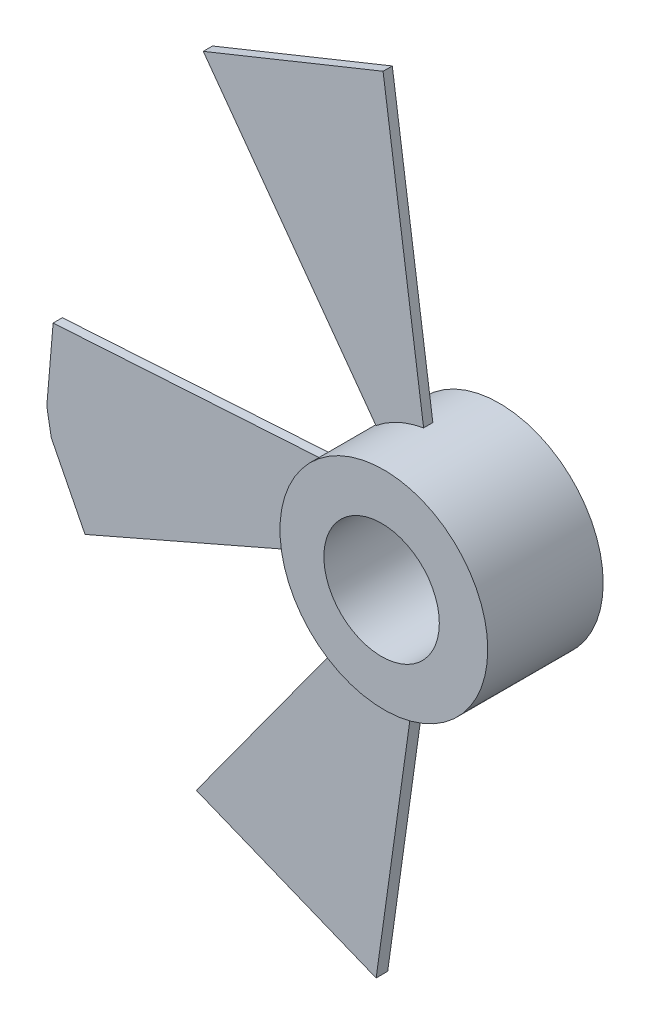
SolidWorks part; units mm, degrees
ref_plane "前视基准面" through (0, 0, 0) normal (0, 0, 1) x (1, 0, 0)
ref_plane "上视基准面" through (0, 0, 0) normal (0, 1, 0) x (1, 0, 0)
ref_plane "右视基准面" through (0, 0, 0) normal (1, 0, 0) x (0, 0, -1)
other "Configuration Table"
sketch "草图1" plane through (0, 0, 0) normal (0, 0, 1) x (1, 0, 0)
  line L0 (-10.9248, 55.6689) -> (-50.6906, 338.617)
  line L1 (-50.6906, 338.617) -> (-206.438, 275.691)
  line L2 (-206.438, 275.691) -> (-37.9182, 43.7433)
  line L9 (-341.9666, -58.1608) -> (-338.1462, -79.9147)
  line L10 (-338.1462, -79.9147) -> (-308.8391, -137.9328)
  line L12 (-308.8391, -137.9328) -> (-53.4903, -26.6467)
  line L13 (11.4967, -2.8593) -> (11.4967, 92.3028) construction
  line L14 (-53.4903, 24.3899) -> (-336.5084, 6.8392)
  line L16 (-341.9666, -58.1608) -> (-336.5084, 6.8392)
  line L17 (-14.9774, -57.1362) -> (-46.9629, -340)
  line L18 (-46.9629, -340) -> (68.0371, -340)
  line L20 (68.0371, -340) -> (24.7526, -52.0453)
  arc A5 (-53.4903, 24.3899) -> (-53.4903, -26.6467) centre (-1.9629, -1.1284) ccw
  arc A7 (-10.9248, 55.6689) -> (-37.9182, 43.7433) centre (-1.9629, -1.1284) ccw
  arc A8 (-14.9774, -57.1362) -> (24.7526, -52.0453) centre (-1.9629, -1.1284) ccw
  point P25 (-59.4629, -1.1284)
  dimension "D2" = 115
  dimension "D1" = 65
  dimension "D3" = 8
  dimension "D4" = 28
  dimension "D5" = 65
  dimension "D6" = 20
  dimension "D7" = 15
  dimension "D8" = 60
  dimension "D9" = 45
extrude "凸台-拉伸1" add sketch "草图1" along normal mid plane 8
sketch "草图2" plane through (0, 0, 4) normal (0, 0, 1) x (1, 0, 0)
  arc A0 (-10.9248, 55.6689) -> (-37.9182, 43.7433) centre (-1.9629, -1.1284) ccw construction
  circle A1 centre (-1.9629, -1.1284) radius 57.5
  circle A2 centre (0, 0) radius 90
  dimension "D1" = 180
extrude "凸台-拉伸2" add sketch "草图2" along normal mid plane 100
sketch "草图3" plane through (0, 0, 0) normal (1, 0, 0) x (0, 0, -1)
  line L0 (0, 0) -> (-54, 0)
  line L1 (-54, 90) -> (-54, -90) construction
sketch "草图4" plane through (0, 0, 54) normal (0, 0, 1) x (1, 0, 0)
  circle A0 centre (-1.9629, -1.1284) radius 57.5 construction
  circle A1 centre (-1.9629, -1.1284) radius 57.5
  circle A2 centre (-1.9629, -1.1284) radius 50
  dimension "D1" = 100
extrude "凸台-拉伸3" add sketch "草图4" against normal blind 100
sketch "草图7" plane through (0, 0, 4) normal (0, 0, 1) x (1, 0, 0)
  line L3 (-18.4767, -88.083) -> (-46.9629, -340)
  line L4 (-46.9629, -340) -> (68.0371, -340)
  line L5 (68.0371, -340) -> (29.7, -84.9583)
  line L6 (-18.4767, -88.083) -> (-46.9629, -340)
  line L7 (-46.9629, -340) -> (68.0371, -340)
  line L8 (68.0371, -340) -> (29.7, -84.9583)
  arc A1 (-18.4767, -88.083) -> (29.7, -84.9583) centre (0, 0) ccw
  arc A2 (-18.4767, -88.083) -> (29.7, -84.9583) centre (0, 0) ccw
  dimension "D1" = 0
extrude "切除-拉伸1" cut sketch "草图7" against normal through all
sketch "草图8" [suppressed] plane through (0, 0, 4) normal (0, 0, 1) x (1, 0, 0)
  line L0 (-57.6509, -69.1113) -> (-212.6596, -244.616)
  line L1 (-212.6596, -244.616) -> (-126.9751, -320.2939)
  line L2 (-126.9751, -320.2939) -> (-11.9985, -89.1966)
  line L3 (-308.8391, -137.9328) -> (-81.2361, -38.7389) construction
  circle A1 centre (0, 0) radius 90
  arc A2 (-57.6509, -69.1113) -> (-11.9985, -89.1966) centre (0, 0) ccw
  point P6 (-108.4639, -303.7978)
  point P9 (-126.9751, -320.2939)
  dimension "D2" = 25
  dimension "D3" = 15
  dimension "D1" = 0
sketch "草图9" plane through (0, 0, 0) normal (0, 0, 1) x (1, 0, 0)
  line L0 (0, 0) -> (199.9805, 0) construction
  line L1 (-206.438, -275.691) -> (-56.8367, -69.7824)
  line L2 (-50.6906, -338.617) -> (-206.438, -275.691)
  line L3 (-15.5593, 88.6448) -> (-50.6906, 338.617)
  line L4 (-50.6906, 338.617) -> (-206.438, 275.691)
  line L5 (-206.438, 275.691) -> (-56.8367, 69.7824)
  line L6 (-15.5593, 88.6448) -> (-50.6906, 338.617) construction
  line L7 (-50.6906, 338.617) -> (-206.438, 275.691) construction
  line L8 (-206.438, 275.691) -> (-56.8367, 69.7824) construction
  line L9 (-15.5593, -88.6448) -> (-50.6906, -338.617)
  arc A0 (-15.5593, -88.6448) -> (-56.8367, -69.7824) centre (0, 0) cw
  arc A1 (-15.5593, 88.6448) -> (-56.8367, 69.7824) centre (0, 0) ccw
  arc A2 (-15.5593, 88.6448) -> (-56.8367, 69.7824) centre (0, 0) ccw construction
  point P5 (0, 0)
  point P7 (0, 0)
  dimension "D1" = 0
extrude "凸台-拉伸4" add sketch "草图9" along normal blind 10 contours L9 L2 L1 A0
